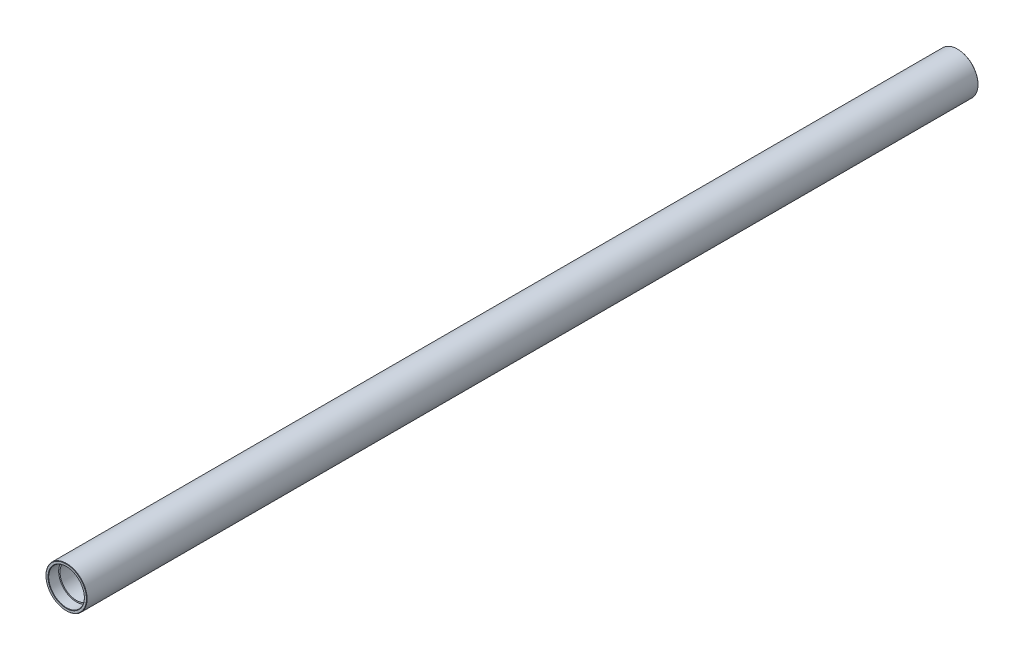
SolidWorks part; units mm, degrees
ref_plane "前视基准面" through (0, 0, 0) normal (0, 0, 1) x (1, 0, 0)
ref_plane "上视基准面" through (0, 0, 0) normal (0, 1, 0) x (1, 0, 0)
ref_plane "右视基准面" through (0, 0, 0) normal (1, 0, 0) x (0, 0, -1)
sketch "草图1" plane through (0, 0, 0) normal (0, 0, 1) x (1, 0, 0)
  circle A0 centre (0, 0) radius 30
  dimension "D1" = 60
extrude "凸台-拉伸1" add sketch "草图1" along normal blind 1300
sketch "草图2" plane through (0, 0, 0) normal (0, 0, -1) x (-1, 0, 0)
  circle A0 centre (0, 0) radius 24
  dimension "D1" = 48
extrude "切除-拉伸1" cut sketch "草图2" against normal blind 1600
sketch "草图3" plane through (0, 0, 0) normal (0, 0, -1) x (-1, 0, 0)
  circle A0 centre (0, 0) radius 26
  dimension "D1" = 52
extrude "切除-拉伸2" cut sketch "草图3" against normal blind 15
sketch "草图4" plane through (0, 0, 1300) normal (0, 0, 1) x (1, 0, 0)
  circle A0 centre (0, 0) radius 26
  dimension "D1" = 52
extrude "切除-拉伸3" cut sketch "草图4" against normal blind 15
chamfer "倒角1" distance 0.5 angle 45 4 edges at (-26, 0, 0) (30, 0, 0) (26, 0, 1300) (30, 0, 1300)
